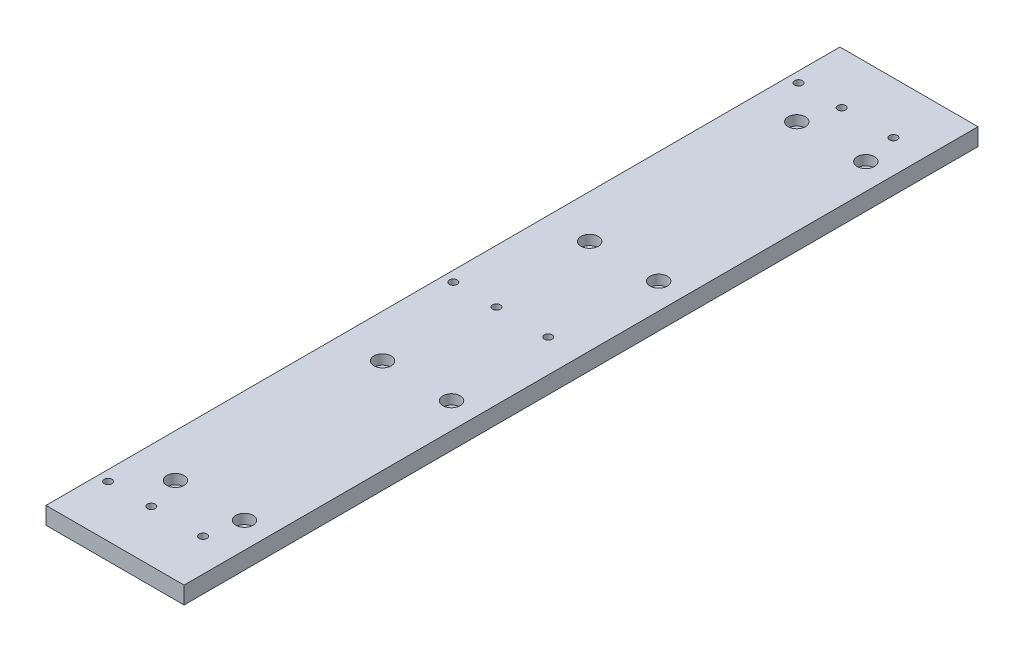
SolidWorks part; units mm, degrees
material "6061 合金"
ref_plane "前视基准面" through (0, 0, 0) normal (0, 0, 1) x (1, 0, 0)
ref_plane "上视基准面" through (0, 0, 0) normal (0, 1, 0) x (1, 0, 0)
ref_plane "右视基准面" through (0, 0, 0) normal (1, 0, 0) x (0, 0, -1)
sketch "草图1" plane through (0, 0, 0) normal (0, 0, 1) x (1, 0, 0)
  line L1 (-40, 5) -> (40, 5)
  line L2 (-40, 5) -> (-40, -5)
  line L3 (-40, -5) -> (40, -5)
  line L4 (40, 5) -> (40, -5)
  line L5 (-40, 5) -> (40, -5) construction
  line L6 (-40, -5) -> (40, 5) construction
  point P0 (0, 0)
  dimension "D1" = 80
  dimension "D2" = 10
extrude "凸台-拉伸1" add sketch "草图1" along normal mid plane 460
hole_wizard "打孔尺寸(%根据)内六角圆柱头螺钉的类型1" positions "草图3" profile "草图2" counterbore size "M4" standard "GB" end condition through all
sketch "草图3" plane through (0, -5, 0) normal (0, -1, 0) x (-1, 0, 0)
  line L0 (40, -230) -> (40, 230) construction
  line L1 (40, -230) -> (-40, -230) construction
  point P0 (34, -200)
  point P2 (9, -200)
  point P4 (-21, -200)
  point P17 (34, 0)
  point P18 (9, 0)
  point P19 (-21, 0)
  point P20 (34, 200)
  point P21 (9, 200)
  point P22 (-21, 200)
  dimension "D1" = 25
  dimension "D2" = 6
  dimension "D3" = 30
  dimension "D4" = 30
  dimension "D5" = 3
sketch "草图2" plane through (-34, -5, 200) normal (1, 0, 0) x (0, 0, -1)
  line L0 (0, 0) -> (0, 10)
  line L1 (0, 10) -> (2.25, 10)
  line L3 (2.25, 10) -> (2.25, 4.6)
  line L4 (2.25, 4.6) -> (4, 4.6)
  line L5 (4, 4.6) -> (4, 0)
  line L7 (4, 0) -> (0, 0)
  line L11 (0, -6.35) -> (0, 107.95) construction
  dimension "通孔孔直径" = 4.5
  dimension "通孔孔深度" = 10
  dimension "柱形沉头孔直径" = 8
  dimension "柱形沉头孔深度" = 4.6
hole_wizard "打孔尺寸(%根据)内六角圆柱头螺钉的类型2" positions "草图5" profile "草图4" counterbore size "M5" standard "GB" end condition through all
sketch "草图5" plane through (0, 5, 0) normal (0, 1, 0) x (1, 0, 0)
  line L1 (40, -230) -> (40, 230) construction
  point P0 (-15, -180)
  point P2 (25, -180)
  point P4 (-15, -60)
  point P6 (25, -60)
  point P8 (25, 60)
  point P10 (25, 180)
  point P12 (-15, 180)
  point P14 (-15, 60)
  dimension "D1" = 120
  dimension "D2" = 120
  dimension "D3" = 120
  dimension "D4" = 60
  dimension "D5" = 40
  dimension "D6" = 15
sketch "草图4" plane through (-15, 5, 180) normal (1, 0, 0) x (0, 0, 1)
  line L0 (0, 0) -> (0, 10)
  line L1 (0, 10) -> (2.75, 10)
  line L3 (2.75, 10) -> (2.75, 5.7)
  line L4 (2.75, 5.7) -> (5, 5.7)
  line L5 (5, 5.7) -> (5, 0)
  line L7 (5, 0) -> (0, 0)
  line L11 (0, -6.35) -> (0, 107.95) construction
  dimension "通孔孔直径" = 5.5
  dimension "通孔孔深度" = 10
  dimension "柱形沉头孔直径" = 10
  dimension "柱形沉头孔深度" = 5.7
